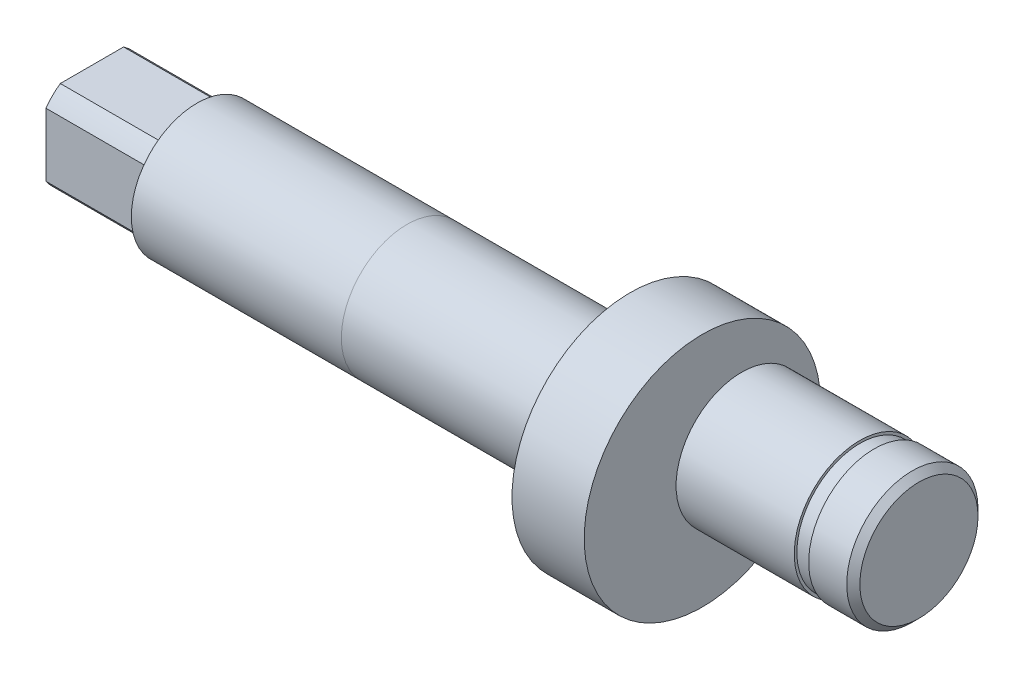
from build123d import *

# Parameters (mm, degrees)
SKETCH_2_R      = 9
EXTRUDE_1_DEPTH = 5.5
SKETCH_3_R      = 5
EXTRUDE_2_DEPTH = 9
SKETCH_4_R      = 4.8
EXTRUDE_3_DEPTH = 1.1
SKETCH_5_R      = 5
EXTRUDE_4_DEPTH = 3.4
CHAMFER_1_SIZE  = 0.5
SKETCH_6_R      = 5
EXTRUDE_5_DEPTH = 17
SKETCH_7_R      = 5
EXTRUDE_6_DEPTH = 16
EXTRUDE_7_DEPTH = 8


with BuildPart() as part:
    # 草图2 → 凸台-拉伸1 (new body)
    with BuildSketch(Plane(origin=(0, 0, 0), x_dir=(0, 0, -1), z_dir=(1, 0, 0))):
        Circle(SKETCH_2_R)
    extrude(amount=EXTRUDE_1_DEPTH)

    # 草图3 → 凸台-拉伸2 (add)
    with BuildSketch(Plane(origin=(5.5, 0, 0), x_dir=(0, 0, -1), z_dir=(1, 0, 0))):
        with Locations((3, 0)):
            Circle(SKETCH_3_R)
    extrude(amount=EXTRUDE_2_DEPTH)

    # 草图4 → 凸台-拉伸3 (add)
    with BuildSketch(Plane(origin=(14.5, 0, 0), x_dir=(0, 0, -1), z_dir=(1, 0, 0))):
        with Locations((3, 0)):
            Circle(SKETCH_4_R)
    extrude(amount=EXTRUDE_3_DEPTH)

    # 草图5 → 凸台-拉伸4 (add)
    with BuildSketch(Plane(origin=(15.6, 0, 0), x_dir=(0, 0, -1), z_dir=(1, 0, 0))):
        with Locations((3, 0)):
            Circle(SKETCH_5_R)
    extrude(amount=EXTRUDE_4_DEPTH)

    # 倒角1
    chamfer_1_edges = [part.edges().sort_by_distance(p)[0] for p in [
        (19, 0, 2),
    ]]
    chamfer(chamfer_1_edges, length=CHAMFER_1_SIZE)

    # 草图6 → 凸台-拉伸5 (add)
    with BuildSketch(Plane.ZY):
        Circle(SKETCH_6_R)
    extrude(amount=EXTRUDE_5_DEPTH)


with BuildPart() as body_2:
    # 草图7 → 凸台-拉伸6 (new body)
    with BuildSketch(Plane.ZY.offset(17)):
        Circle(SKETCH_7_R)
    extrude(amount=EXTRUDE_6_DEPTH)

    # 草图8 → 凸台-拉伸7 (add)
    with BuildSketch(Plane.ZY.offset(33)):
        with BuildLine():
            Line((-2.41091269, -3.5), (2.41091269, -3.5))
            ThreePointArc((2.41091269, -3.5), (3.00520382, -3.00520382), (3.5, -2.41091269))
            Line((3.5, -2.41091269), (3.5, 2.41091269))
            ThreePointArc((3.5, 2.41091269), (3.00520382, 3.00520382), (2.41091269, 3.5))
            Line((2.41091269, 3.5), (-2.41091269, 3.5))
            ThreePointArc((-2.41091269, 3.5), (-3.00520382, 3.00520382), (-3.5, 2.41091269))
            Line((-3.5, 2.41091269), (-3.5, -2.41091269))
            ThreePointArc((-3.5, -2.41091269), (-3.00520382, -3.00520382), (-2.41091269, -3.5))
        make_face()
    extrude(amount=EXTRUDE_7_DEPTH)


solid = Compound([part.part, body_2.part])
